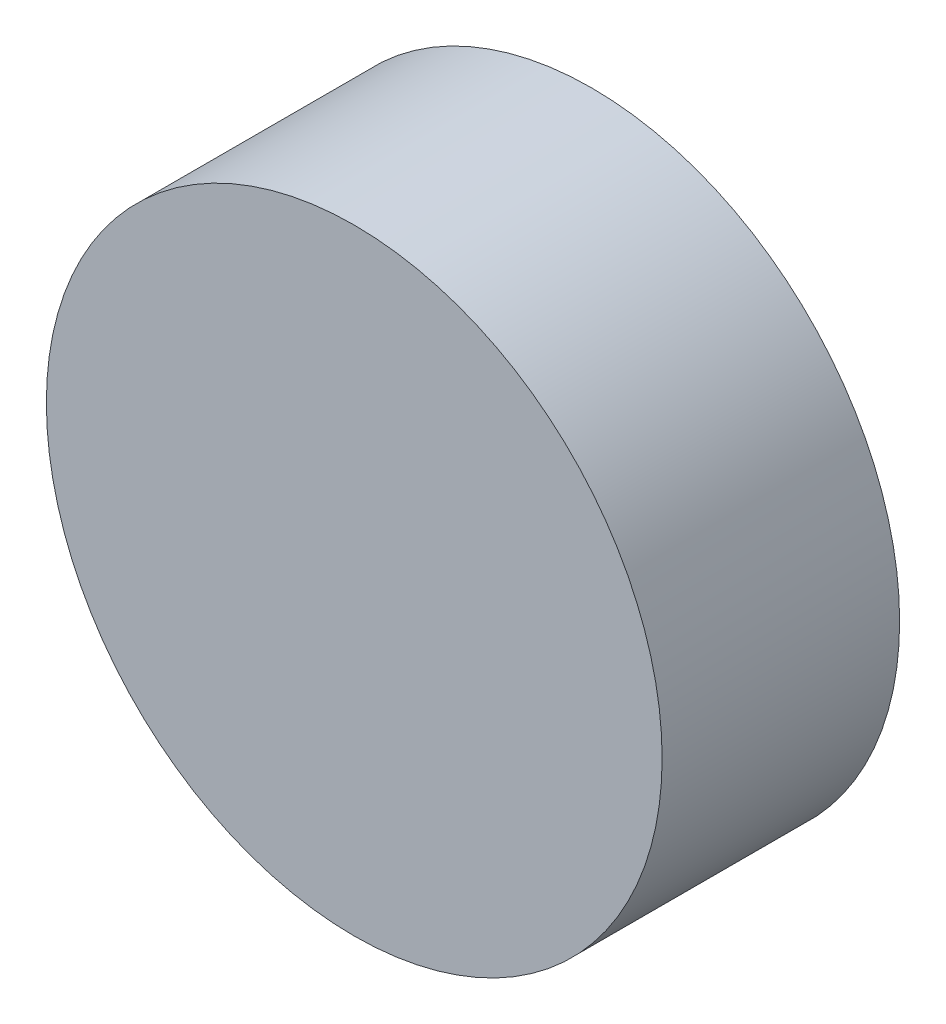
from build123d import *

# Parameters (mm, degrees)
SKETCH1_R           = 12.963501109
BOSS_EXTRUDE1_DEPTH = 10


with BuildPart() as part:
    # Sketch1 → Boss-Extrude1 (new body)
    with BuildSketch(Plane.XY):
        with Locations((-17.055797946, 0)):
            Circle(SKETCH1_R)
    extrude(amount=BOSS_EXTRUDE1_DEPTH)


solid = part.part
